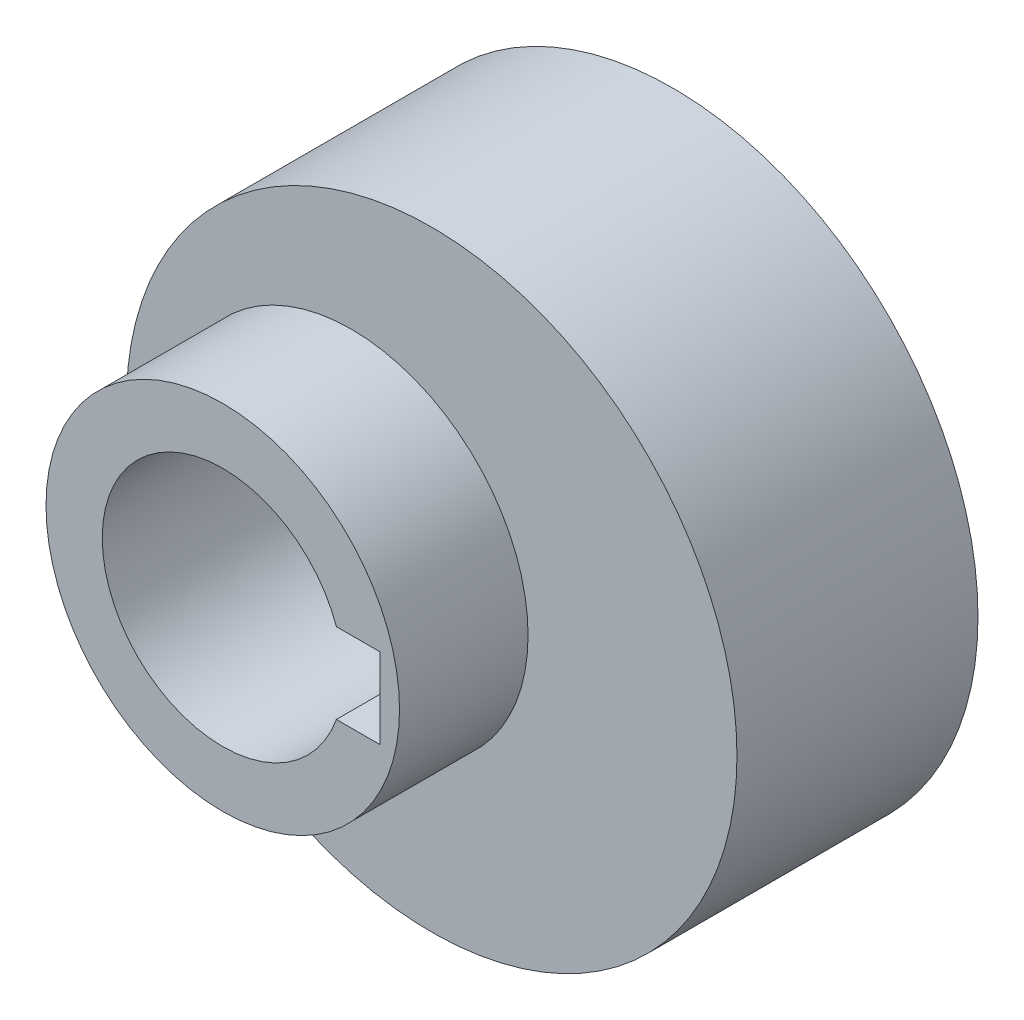
from build123d import *

# Parameters (mm, degrees)
SKETCH1_R           = 11
BOSS_EXTRUDE1_DEPTH = 26
BOSS_EXTRUDE2_START = -8
SKETCH2_R           = 19
BOSS_EXTRUDE2_DEPTH = 15
CUT_EXTRUDE1_DEPTH  = 43


with BuildPart() as part:
    # Sketch1 → Boss-Extrude1 (new body)
    with BuildSketch(Plane.XY):
        with Locations(Location((0, 0, 0), (0, 0, 180))):
            Circle(SKETCH1_R)
    extrude(amount=BOSS_EXTRUDE1_DEPTH)

    # Sketch2 → Boss-Extrude2 (add)
    with BuildSketch(Plane.XY.offset(26).offset(BOSS_EXTRUDE2_START)):
        with Locations((5, 0)):
            Circle(SKETCH2_R)
    extrude(amount=-BOSS_EXTRUDE2_DEPTH)

    # Sketch3 → Cut-Extrude1 (cut)
    with BuildSketch(Plane.XY.offset(26)):
        with BuildLine():
            Line((7.071067812, 2.5), (9.8, 2.5))
            Line((9.8, 2.5), (9.8, -2.5))
            Line((9.8, -2.5), (7.071067812, -2.5))
            ThreePointArc((7.071067812, -2.5), (-7.5, 0), (7.071067812, 2.5))
        make_face()
    extrude(amount=-CUT_EXTRUDE1_DEPTH, mode=Mode.SUBTRACT)


solid = part.part
